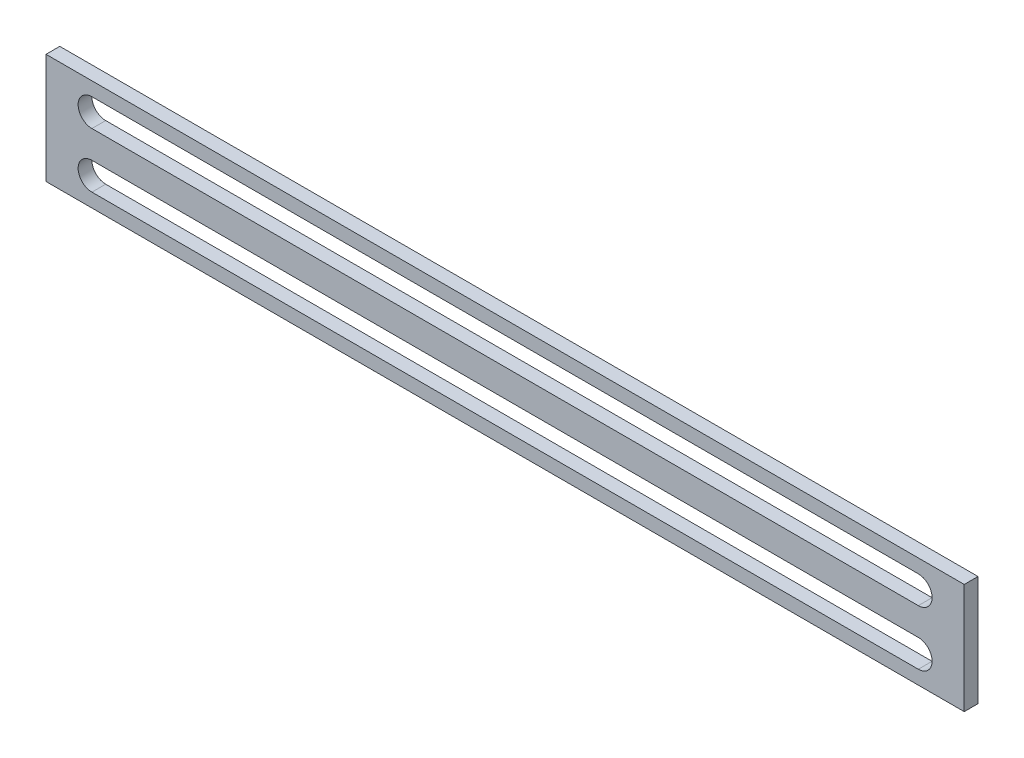
from build123d import *

# Parameters (mm, degrees)
SKETCH_1_W      = 100
SKETCH_1_H      = 12
EXTRUDE_1_DEPTH = 1.5


with BuildPart() as part:
    # 草图1 → 凸台-拉伸1 (new body)
    with BuildSketch(Plane.XY):
        Rectangle(SKETCH_1_W, SKETCH_1_H)
        with BuildLine():
            Line((-45, 4.5), (45, 4.5))
            ThreePointArc((45, 4.5), (46.5, 3), (45, 1.5))
            Line((45, 1.5), (-45, 1.5))
            ThreePointArc((-45, 1.5), (-46.5, 3), (-45, 4.5))
        make_face(mode=Mode.SUBTRACT)
        with BuildLine():
            Line((-45, -4.5), (45, -4.5))
            ThreePointArc((45, -4.5), (46.5, -3), (45, -1.5))
            Line((45, -1.5), (-45, -1.5))
            ThreePointArc((-45, -1.5), (-46.5, -3), (-45, -4.5))
        make_face(mode=Mode.SUBTRACT)
    extrude(amount=EXTRUDE_1_DEPTH)


solid = part.part
